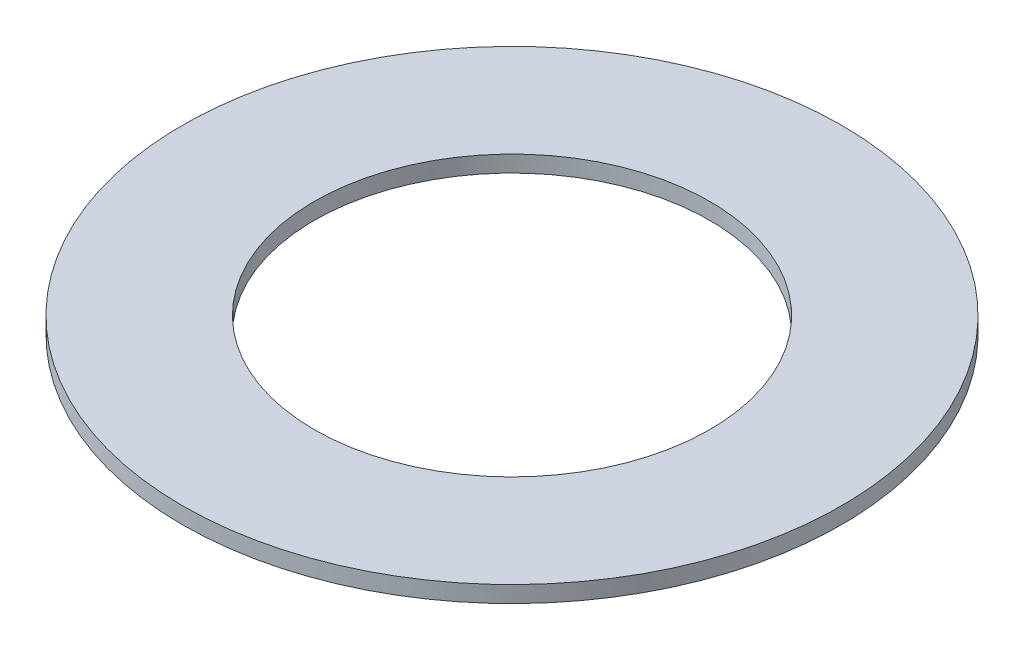
SolidWorks part; units mm, degrees
material "AISI 304"
ref_plane "前视基准面" through (0, 0, 0) normal (0, 0, 1) x (1, 0, 0)
ref_plane "上视基准面" through (0, 0, 0) normal (0, 1, 0) x (1, 0, 0)
ref_plane "右视基准面" through (0, 0, 0) normal (1, 0, 0) x (0, 0, -1)
sketch "草图1" plane through (0, 0, 0) normal (0, 1, 0) x (1, 0, 0)
  circle A0 centre (0, 0) radius 10
  circle A1 centre (0, 0) radius 6
  dimension "D1" = 20
  dimension "D2" = 12
extrude "凸台-拉伸1" add sketch "草图1" along normal blind 0.5
